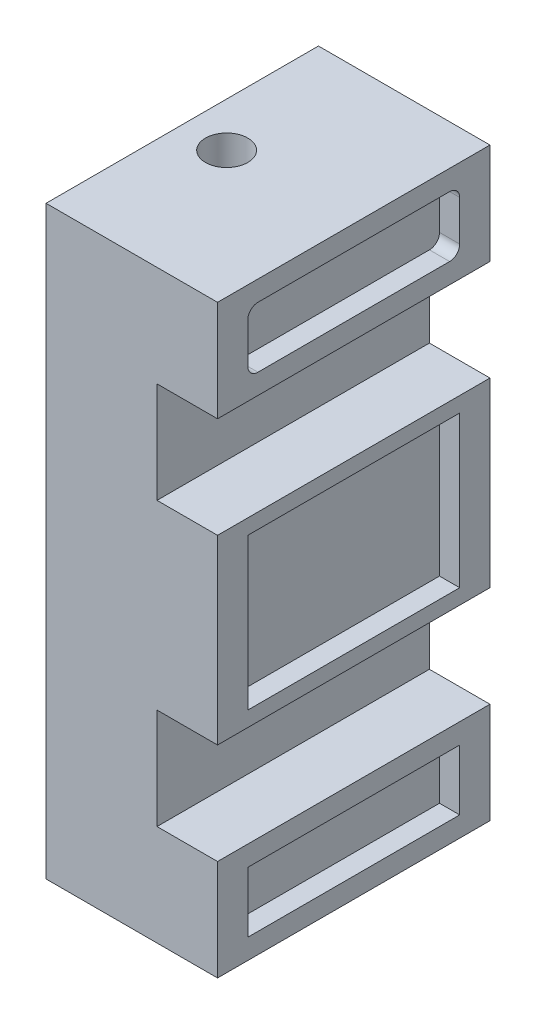
from build123d import *

# Parameters (mm, degrees)
EXTRUDE_1_DEPTH        = 13.5
SKETCH_2_W             = 21
SKETCH_2_H             = 6
SKETCH_2_H_2           = 15
CUT_EXTRUDE_1_DEPTH    = 2
FILLET_1_R             = 1
SKETCH_3_R             = 2.1
CUT_EXTRUDE_2_DEPTH    = 58
HOLE_WIZARD_M5_1_D     = 4.2
HOLE_WIZARD_M5_1_DEPTH = 8
HOLE_WIZARD_M5_1_TIP   = 1.2618073


with BuildPart() as part:
    # 草图1 → 凸台-拉伸1 (new, symmetric)
    with BuildSketch(Plane.XY):
        Polygon((0, 0), (0, 29), (17, 29), (17, 19), (11, 19), (11, 9), (17, 9), (17, -9), (11, -9), (11, -19), (17, -19), (17, -29), (0, -29), align=None)
    extrude(amount=EXTRUDE_1_DEPTH, both=True)

    # 草图2 → 切除-拉伸1 (cut)
    with BuildSketch(Plane(origin=(17, 0, 0), x_dir=(0, 0, -1), z_dir=(1, 0, 0))):
        with Locations((0, 24)):
            Rectangle(SKETCH_2_W, SKETCH_2_H)
        Rectangle(SKETCH_2_W, SKETCH_2_H_2)
        with Locations((0, -24)):
            Rectangle(SKETCH_2_W, SKETCH_2_H)
    extrude(amount=-CUT_EXTRUDE_1_DEPTH, mode=Mode.SUBTRACT)

    # 圆角1
    fillet_1_edges = [part.edges().sort_by_distance(p)[0] for p in [
        (16, 27, -10.5),
        (16, 21, -10.5),
        (16, 21, 10.5),
        (16, 27, 10.5),
    ]]
    fillet(fillet_1_edges, radius=FILLET_1_R)

    # 草图3 → 切除-拉伸2 (cut)
    with BuildSketch(Plane(origin=(0, 29, 0), x_dir=(1, 0, 0), z_dir=(0, 1, 0))):
        with Locations(Location((4.4, 0, 0), (0, 0, 180))):
            Circle(SKETCH_3_R)
    extrude(amount=-CUT_EXTRUDE_2_DEPTH, mode=Mode.SUBTRACT)

    # M5 螺纹孔1
    with Locations(Plane(origin=(4.4, 29, 0), x_dir=(0, 0, 1), z_dir=(0, 1, 0))):
        with Locations((0, 0)):
            Hole(HOLE_WIZARD_M5_1_D / 2, depth=HOLE_WIZARD_M5_1_DEPTH)
            with Locations((0, 0, -(HOLE_WIZARD_M5_1_DEPTH + HOLE_WIZARD_M5_1_TIP / 2))):  # 118° drill point
                Cone(0, HOLE_WIZARD_M5_1_D / 2, HOLE_WIZARD_M5_1_TIP, mode=Mode.SUBTRACT)


solid = part.part
